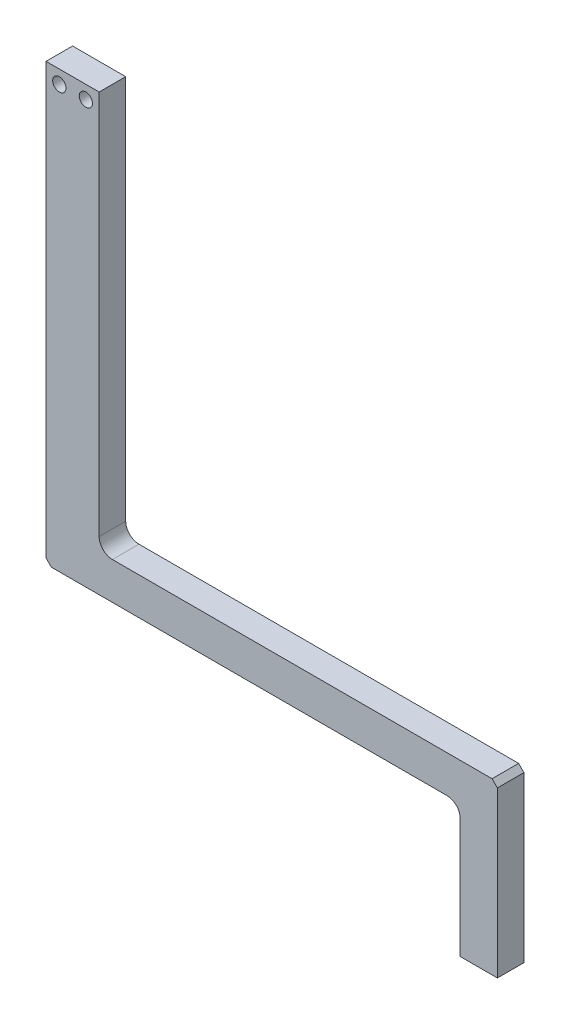
SolidWorks part; units mm, degrees
ref_plane "前视基准面" through (0, 0, 0) normal (0, 0, 1) x (1, 0, 0)
ref_plane "上视基准面" through (0, 0, 0) normal (0, 1, 0) x (1, 0, 0)
ref_plane "右视基准面" through (0, 0, 0) normal (1, 0, 0) x (0, 0, -1)
sketch "草图1" plane through (0, 0, 0) normal (0, 0, 1) x (1, 0, 0)
  line L0 (0, 0) -> (-85, 0)
  line L3 (-85, 0) -> (-85, 164)
  line L4 (-85, 164) -> (-65, 164)
  line L5 (-65, 164) -> (-65, 14)
  line L6 (-65, 14) -> (85, 14)
  line L7 (85, 14) -> (85, 0)
  line L8 (85, 0) -> (0, 0)
  dimension "D1" = 150
  dimension "D2" = 20
  dimension "D3" = 14
  dimension "D4" = 150
extrude "凸台-拉伸1" add sketch "草图1" along normal mid plane 10
sketch "草图2" plane through (0, 0, 5) normal (0, 0, 1) x (1, 0, 0)
  line L0 (-65, 164) -> (-85, 164) construction
  line L1 (-65, 14) -> (-65, 164) construction
  line L2 (-85, 164) -> (-85, 0) construction
  circle A0 centre (-80, 159) radius 2.5
  circle A1 centre (-70, 159) radius 2.5
  dimension "D2" = 5
  dimension "D1" = 5
  dimension "D3" = 5
  dimension "D4" = 5
extrude "切除-拉伸1" cut sketch "草图2" against normal up to next
sketch "草图3" plane through (0, 0, 5) normal (0, 0, 1) x (1, 0, 0)
  line L1 (85, 0) -> (71, 0)
  line L2 (85, 0) -> (85, -50)
  line L3 (85, -50) -> (71, -50)
  line L4 (71, 0) -> (71, -50)
  dimension "D1" = 14
  dimension "D2" = 50
extrude "凸台-拉伸2" add sketch "草图3" against normal up to surface (10 mm away) up to face at (-82.5, 159, -5)
fillet "圆角1" radius 5 2 edges at (-65, 14, 0) (71, 0, 0)
chamfer "倒角1" distance 2 angle 45 2 edges at (-85, 0, 0) (85, 14, 0)
